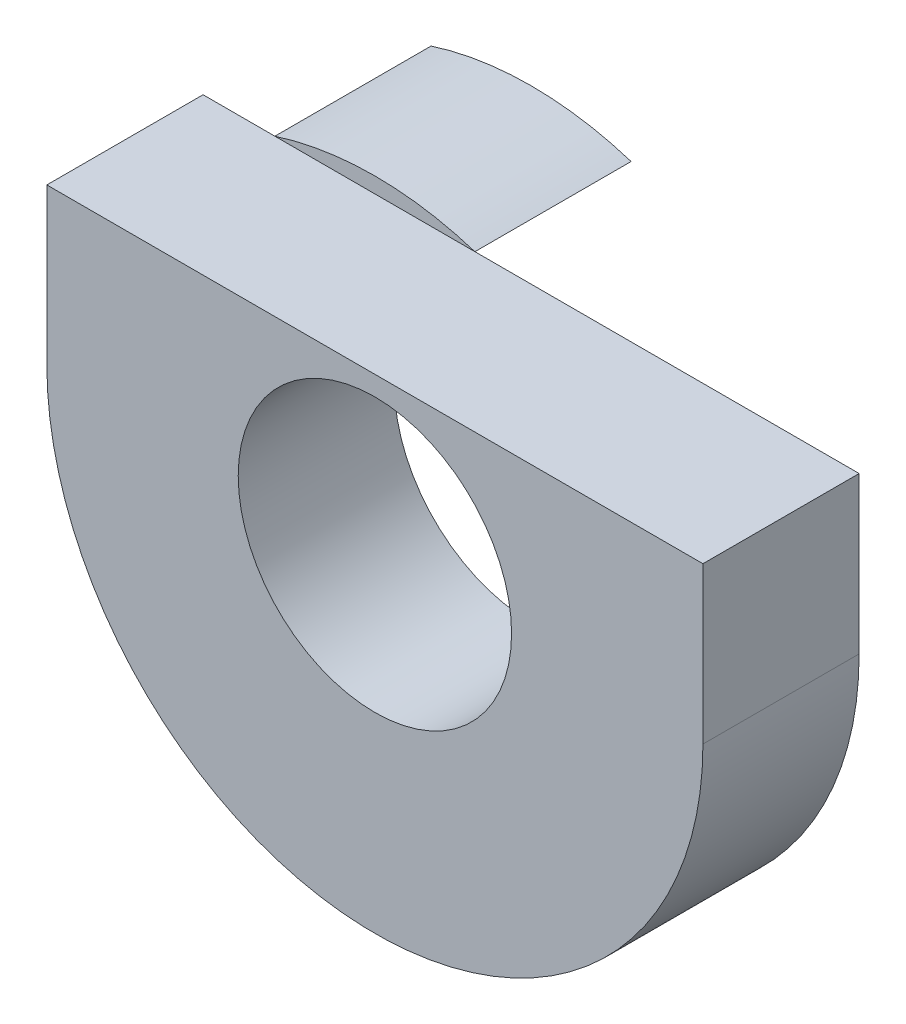
from build123d import *

# Parameters (mm, degrees)
SKETCH1_R           = 210
SKETCH1_R_2         = 87.5
BOSS_EXTRUDE1_DEPTH = 100
BOSS_EXTRUDE2_START = -100
BOSS_EXTRUDE2_DEPTH = 100
SKETCH3_W           = 369.323706252
SKETCH3_H           = 100
CUT_EXTRUDE1_DEPTH  = 314.36879232


with BuildPart() as part:
    # Sketch1 → Boss-Extrude1 (new body)
    with BuildSketch(Plane.XY):
        Circle(SKETCH1_R)
        Circle(SKETCH1_R_2, mode=Mode.SUBTRACT)
    extrude(amount=BOSS_EXTRUDE1_DEPTH)

    # Sketch2 → Boss-Extrude2 (add)
    with BuildSketch(Plane.XY.offset(100).offset(BOSS_EXTRUDE2_START)):
        with BuildLine():
            Line((87.5, 0), (210, 0))
            Line((210, 0), (210, 100))
            Line((210, 100), (-210, 100))
            Line((-210, 100), (-210, 0))
            Line((-210, 0), (-87.5, 0))
            ThreePointArc((-87.5, 0), (0, 87.5), (87.5, 0))
        make_face()
    extrude(amount=BOSS_EXTRUDE2_DEPTH)

    # Sketch3 → Cut-Extrude1 (cut, through all)
    with BuildSketch(Plane(origin=(0, 0, 0), x_dir=(-1, 0, 0), z_dir=(0, 0, -1))):
        with Locations((0, 150)):
            Rectangle(SKETCH3_W, SKETCH3_H)
    extrude(amount=-CUT_EXTRUDE1_DEPTH, mode=Mode.SUBTRACT)


with BuildPart() as cut_extrude1_piece_1:
    # of the separate pieces the step leaves, piece 1, a body of its own (cut_extrude1_pieces)
    add(part.part.solids().sort_by_distance((-210, 100, 0))[0])


with BuildPart() as cut_extrude1_piece_2:
    # of the separate pieces the step leaves, piece 2, a body of its own (cut_extrude1_pieces)
    add(part.part.solids().sort_by_distance((64.031242374, 200, 0))[0])


solid = Compound([cut_extrude1_piece_1.part, cut_extrude1_piece_2.part])
